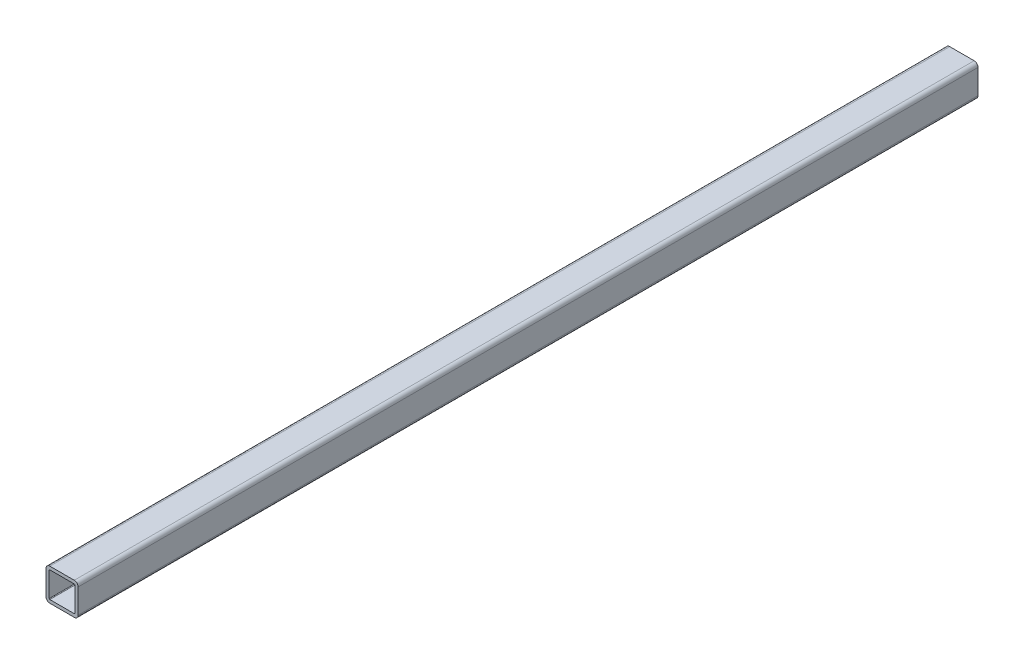
SolidWorks part; units mm, degrees
material "Q235B"
ref_plane "Front Plane" through (0, 0, 0) normal (0, 0, 1) x (1, 0, 0)
ref_plane "Top Plane" through (0, 0, 0) normal (0, 1, 0) x (1, 0, 0)
ref_plane "Right Plane" through (0, 0, 0) normal (1, 0, 0) x (0, 0, -1)
sketch "Sketch1" plane through (0, 0, 0) normal (0, 0, 1) x (1, 0, 0)
  line L0 (6, 45) -> (44, 45)
  line L1 (6, 0) -> (44, 0)
  line L2 (0, 6) -> (0, 44)
  line L3 (6, 50) -> (44, 50)
  line L4 (50, 6) -> (50, 44)
  line L5 (45, 6) -> (45, 44)
  line L6 (6, 5) -> (44, 5)
  line L7 (5, 6) -> (5, 44)
  arc A0 (6, 0) -> (0, 6) centre (6, 6) cw
  arc A1 (44, 0) -> (50, 6) centre (44, 6) ccw
  arc A2 (44, 50) -> (50, 44) centre (44, 44) cw
  arc A3 (0, 44) -> (6, 50) centre (6, 44) cw
  arc A4 (5, 44) -> (6, 45) centre (6, 44) cw
  arc A5 (44, 45) -> (45, 44) centre (44, 44) cw
  arc A6 (44, 5) -> (45, 6) centre (44, 6) ccw
  arc A7 (6, 5) -> (5, 6) centre (6, 6) cw
  point P7 (0, 0)
  point P12 (50, 50)
  point P15 (0, 50)
  dimension "D3" = 6
  dimension "D1" = 50
  dimension "D2" = 50
  dimension "D4" = 5
extrude "Boss-Extrude1" add sketch "Sketch1" along normal blind 1400
